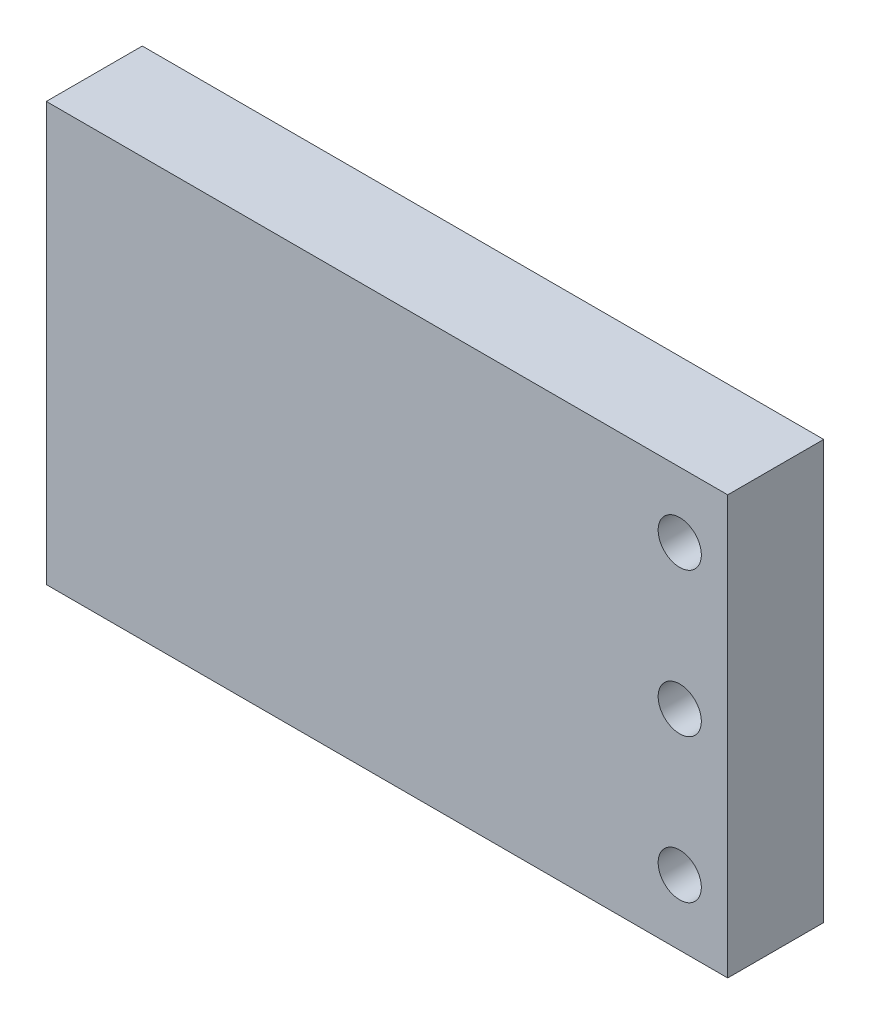
SolidWorks part; units mm, degrees
ref_plane "前视基准面" through (0, 0, 0) normal (0, 0, 1) x (1, 0, 0)
ref_plane "上视基准面" through (0, 0, 0) normal (0, 1, 0) x (1, 0, 0)
ref_plane "右视基准面" through (0, 0, 0) normal (1, 0, 0) x (0, 0, -1)
sketch "草图1" plane through (0, 0, 0) normal (0, 1, 0) x (1, 0, 0)
  line L1 (0, 0) -> (71, 0)
  line L2 (0, 0) -> (0, 10)
  line L3 (0, 10) -> (71, 10)
  line L4 (71, 0) -> (71, 10)
  dimension "D1" = 10
  dimension "D2" = 71
extrude "凸台-拉伸1" add sketch "草图1" along normal blind 43.6
sketch "草图4" plane through (0, 0, -10) normal (0, 0, -1) x (-1, 0, 0)
  line L0 (0, 21.8) -> (-89.3798, 21.8) construction
  line L1 (0, 43.6) -> (0, 0) construction
  line L3 (-71, 43.6) -> (-71, 0) construction
  point P0 (-66, 36.8)
  point P2 (-66, 21.7835)
  point P4 (-66, 6.8)
  dimension "D1" = 30
  dimension "D2" = 5
hole_wizard "M4 六角圆柱头螺钉的柱形沉头孔1" positions "草图4" profile "草图3" counterbore size "M4" standard "GB" end condition through all
sketch "草图3" plane through (66, 36.8, -10) normal (1, 0, 0) x (0, 1, 0)
  line L0 (0, 0) -> (0, 10)
  line L1 (0, 10) -> (2.25, 10)
  line L3 (2.25, 10) -> (2.25, 4.6)
  line L4 (2.25, 4.6) -> (4, 4.6)
  line L5 (4, 4.6) -> (4, 0)
  line L7 (4, 0) -> (0, 0)
  line L11 (0, -6.35) -> (0, 107.95) construction
  dimension "通孔孔直径" = 4.5
  dimension "通孔孔深度" = 10
  dimension "柱形沉头孔直径" = 8
  dimension "柱形沉头孔深度" = 4.6
sketch "草图7" plane through (0, 0, 0) normal (-1, 0, 0) x (0, 0, 1)
  point P0 (-5, 37.8)
  point P3 (-5, 21.8)
  point P6 (-5, 5.8)
hole_wizard "M4 螺纹孔1" positions "草图7" profile "草图6" tap size "M4" standard "GB"
sketch "草图6" plane through (0, 37.8, -5) normal (0, 1, 0) x (0, 0, 1)
  line L0 (0, 0) -> (0, 11.0914)
  line L1 (0, 11.0914) -> (1.65, 10.1)
  line L2 (1.65, 10.1) -> (1.65, 0)
  line L5 (1.65, 0) -> (0, 0)
  line L10 (0, 11.0914) -> (-1.65, 10.1) construction
  line L11 (0, -6.35) -> (0, 107.95) construction
  dimension "螺纹孔钻头直径" = 3.3
  dimension "螺纹孔钻头深度" = 10.1
  dimension "导头角度" = 118
cosmetic thread "孔螺纹线1" parameters "D1"=8, "D2"=4
cosmetic thread "孔螺纹线2" parameters "D1"=8, "D2"=4
cosmetic thread "孔螺纹线3" parameters "D1"=8, "D2"=4
